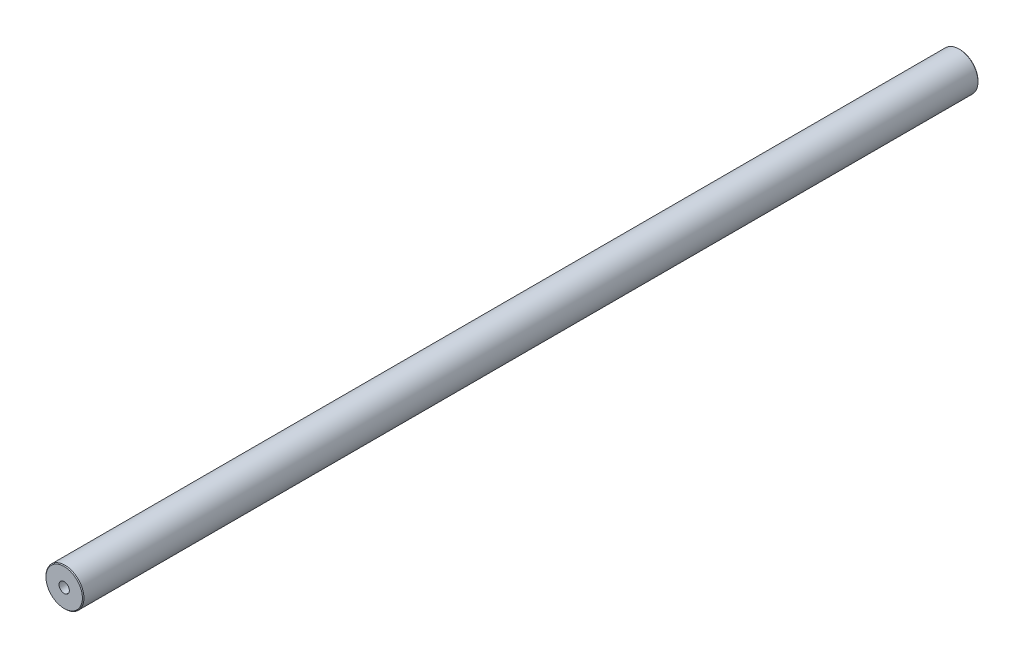
SolidWorks part; units mm, degrees
ref_plane "前视基准面" through (0, 0, 0) normal (0, 0, 1) x (1, 0, 0)
ref_plane "上视基准面" through (0, 0, 0) normal (0, 1, 0) x (1, 0, 0)
ref_plane "右视基准面" through (0, 0, 0) normal (1, 0, 0) x (0, 0, -1)
sketch "草图1" plane through (0, 0, 0) normal (0, 0, 1) x (1, 0, 0)
  circle A0 centre (0, 0) radius 12.5
  dimension "D1" = 25
extrude "凸台-拉伸1" add sketch "草图1" along normal blind 590
hole_wizard "M8 螺纹孔1" positions "草图3" profile "草图2" tap size "M8" standard "ISO"
sketch "草图3" plane through (0, 0, 590) normal (0, 0, 1) x (1, 0, 0)
  point P0 (0, 0)
cosmetic thread "孔螺蚊线1" parameters "D1"=16, "D2"=8
sketch "草图2" plane through (0, 0, 590) normal (1, 0, 0) x (0, -1, 0)
  line L0 (0, 0) -> (0, 21.7929)
  line L1 (0, 21.7929) -> (3.4, 19.75)
  line L2 (3.4, 19.75) -> (3.4, 0)
  line L5 (3.4, 0) -> (0, 0)
  line L10 (0, 21.7929) -> (-3.4, 19.75) construction
  line L11 (0, -6.35) -> (0, 107.95) construction
  dimension "螺纹孔钻头直径" = 6.8
  dimension "螺纹孔钻头深度" = 19.75
  dimension "导头角度" = 118
hole_wizard "M8 螺纹孔2" positions "草图5" profile "草图4" tap size "M8" standard "ISO"
sketch "草图5" plane through (0, 0, 0) normal (0, 0, -1) x (-1, 0, 0)
  point P0 (0, 0)
sketch "草图4" plane through (0, 0, 0) normal (1, 0, 0) x (0, 1, 0)
  line L0 (0, 0) -> (0, 21.7929)
  line L1 (0, 21.7929) -> (3.4, 19.75)
  line L2 (3.4, 19.75) -> (3.4, 0)
  line L5 (3.4, 0) -> (0, 0)
  line L10 (0, 21.7929) -> (-3.4, 19.75) construction
  line L11 (0, -6.35) -> (0, 107.95) construction
  dimension "螺纹孔钻头直径" = 6.8
  dimension "螺纹孔钻头深度" = 19.75
  dimension "导头角度" = 118
cosmetic thread "孔螺蚊线2" parameters "D1"=16, "D2"=8
chamfer "倒角1" distance 0.5 angle 45 3 edges at (12.5, 0, 0) (-3.4, 0, 0) (12.5, 0, 590)
